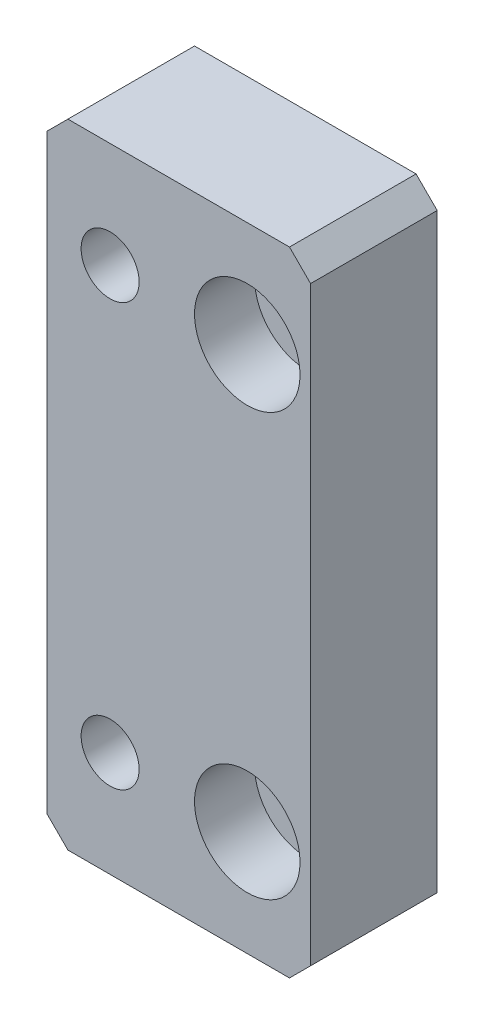
from build123d import *

# Parameters (mm, degrees)
SKETCH_1_W                   = 25
SKETCH_1_H                   = 60
EXTRUDE_1_DEPTH              = 6
CHAMFER_1_SIZE               = 2
HOLE_WIZARD_M5_1_D           = 5.5
HOLE_WIZARD_M5_1_DEPTH       = 12.4
HOLE_WIZARD_M5_1_CBORE_D     = 10
HOLE_WIZARD_M5_1_CBORE_DEPTH = 5.7
HOLE_WIZARD_M5_1_TIP         = 1.652366702
HOLE_WIZARD_M5_2_D           = 5.5
HOLE_WIZARD_M5_2_DEPTH       = 12.4
HOLE_WIZARD_M5_2_CBORE_D     = 10
HOLE_WIZARD_M5_2_CBORE_DEPTH = 5.7
HOLE_WIZARD_M5_2_TIP         = 1.652366702


with BuildPart() as part:
    # 草图1 → 凸台-拉伸1 (new, symmetric)
    with BuildSketch(Plane.XY):
        Rectangle(SKETCH_1_W, SKETCH_1_H)
    extrude(amount=EXTRUDE_1_DEPTH, both=True)

    # 倒角1
    chamfer_1_edges = [part.edges().sort_by_distance(p)[0] for p in [
        (12.5, -30, 0),
        (-12.5, -30, 0),
        (-12.5, 30, 0),
        (12.5, 30, 0),
    ]]
    chamfer(chamfer_1_edges, length=CHAMFER_1_SIZE)

    # M5 六角圆柱头螺钉的柱形沉头孔1
    with Locations(Plane(origin=(0, 0, -6), x_dir=(-1, 0, 0), z_dir=(0, 0, -1))):
        with Locations((6.5, 20), (6.5, -20)):
            CounterBoreHole(HOLE_WIZARD_M5_1_D / 2, HOLE_WIZARD_M5_1_CBORE_D / 2, HOLE_WIZARD_M5_1_CBORE_DEPTH, depth=HOLE_WIZARD_M5_1_DEPTH)
            with Locations((0, 0, -(HOLE_WIZARD_M5_1_DEPTH + HOLE_WIZARD_M5_1_TIP / 2))):  # 118° drill point
                Cone(0, HOLE_WIZARD_M5_1_D / 2, HOLE_WIZARD_M5_1_TIP, mode=Mode.SUBTRACT)

    # M5 六角圆柱头螺钉的柱形沉头孔2
    with Locations(Plane.XY.offset(6)):
        with Locations((6.5, 20), (6.5, -20)):
            CounterBoreHole(HOLE_WIZARD_M5_2_D / 2, HOLE_WIZARD_M5_2_CBORE_D / 2, HOLE_WIZARD_M5_2_CBORE_DEPTH, depth=HOLE_WIZARD_M5_2_DEPTH)
            with Locations((0, 0, -(HOLE_WIZARD_M5_2_DEPTH + HOLE_WIZARD_M5_2_TIP / 2))):  # 118° drill point
                Cone(0, HOLE_WIZARD_M5_2_D / 2, HOLE_WIZARD_M5_2_TIP, mode=Mode.SUBTRACT)


solid = part.part
